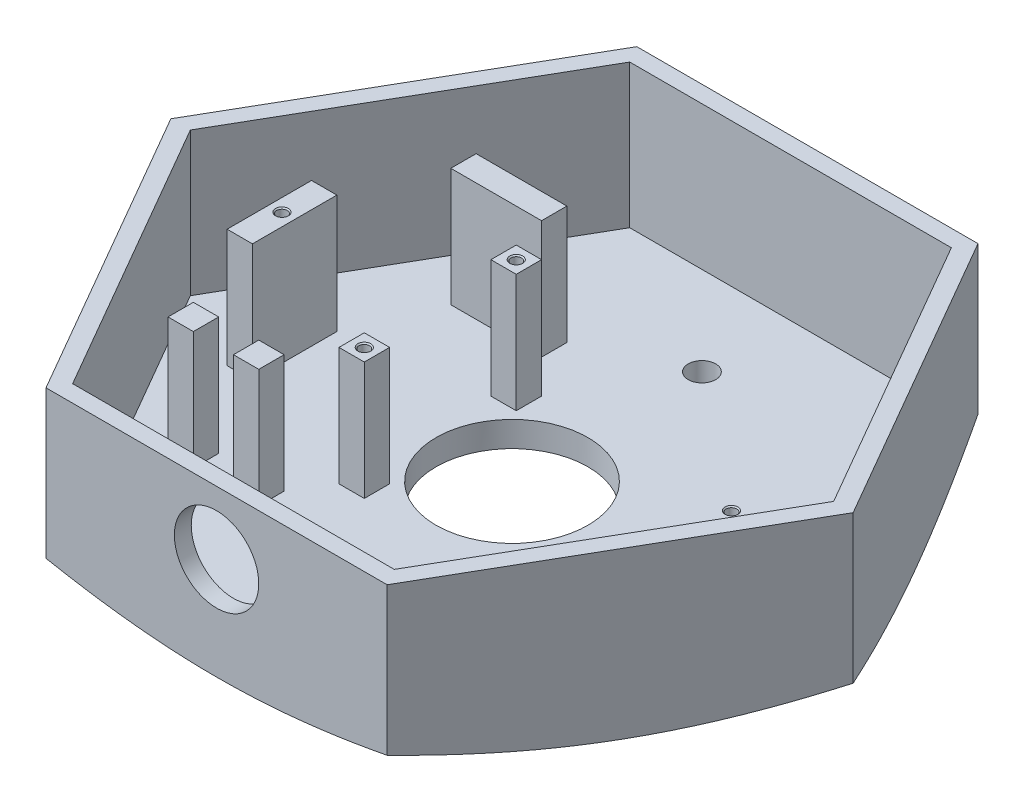
from build123d import *

# Parameters (mm, degrees)
BOSS_EXTRUDE1_DEPTH         = 41
CUT_EXTRUDE1_DEPTH          = 34
SKETCH4_R                   = 52.5
CUT_EXTRUDE2_DEPTH          = 1
SKETCH5_W                   = 21.5
SKETCH5_H                   = 6
SKETCH5_W_2                 = 6
SKETCH5_H_2                 = 20
BOSS_EXTRUDE2_DEPTH         = 28
SKETCH6_R                   = 18
CUT_EXTRUDE3_DEPTH          = 28
SKETCH7_R                   = 3.25
CUT_EXTRUDE4_DEPTH          = 28
M3_TAPPED_HOLE1_D           = 2.5
M3_TAPPED_HOLE1_CSINK_D     = 3.05
M3_TAPPED_HOLE1_CSINK_ANGLE = 90
M3_TAPPED_HOLE2_D           = 2.5
M3_TAPPED_HOLE2_DEPTH       = 8
M3_TAPPED_HOLE2_CSINK_D     = 3.05
M3_TAPPED_HOLE2_CSINK_ANGLE = 90
M3_TAPPED_HOLE2_TIP         = 0.751075774
SKETCH8_R                   = 10
CUT_EXTRUDE5_DEPTH          = 28


with BuildPart() as part:
    # Sketch1 → Boss-Extrude1 (new body)
    with BuildSketch(Plane(origin=(0, 0, 0), x_dir=(1, 0, 0), z_dir=(0, 1, 0))):
        Polygon((-40.414518843, 70), (-80.829037687, 0), (-40.414518843, -70), (40.414518843, -70), (80.829037687, 0), (40.414518843, 70), align=None)
    extrude(amount=BOSS_EXTRUDE1_DEPTH)

    # Sketch2 → Cut-Extrude1 (cut)
    with BuildSketch(Plane(origin=(0, 41, 0), x_dir=(1, 0, 0), z_dir=(0, 1, 0))):
        Polygon((38.105117767, -66), (76.210235533, 0), (38.105117767, 66), (-38.105117767, 66), (-76.210235533, 0), (-38.105117767, -66), align=None)
    extrude(amount=-CUT_EXTRUDE1_DEPTH, mode=Mode.SUBTRACT)

    # Sketch3 → Cut-Revolve1 (revolve, cut)
    with BuildSketch(Plane.XY, mode=Mode.PRIVATE) as cut_revolve1_sk:
        Polygon((-80.829037687, 6), (-65.198503298, 0), (-80.829037687, 0), align=None)
    revolve(cut_revolve1_sk.sketch.rotate(Axis((0, 62.900603769, 0), (0, -1, 0)), 270), axis=Axis((0, 62.900603769, 0), (0, -1, 0)), mode=Mode.SUBTRACT)

    # Sketch4 → Cut-Extrude2 (cut)
    with BuildSketch(Plane.XZ):
        with Locations(Location((0, 0, 0), (0, 0, 270))):
            Circle(SKETCH4_R)
    extrude(amount=-CUT_EXTRUDE2_DEPTH, mode=Mode.SUBTRACT)

    # Sketch5 → Boss-Extrude2 (add)
    with BuildSketch(Plane(origin=(0, 7, 0), x_dir=(1, 0, 0), z_dir=(0, 1, 0))):
        with Locations((-32.75, 32)):
            Rectangle(SKETCH5_W, SKETCH5_H)
        with Locations((-54.5, 0)):
            Rectangle(SKETCH5_W_2, SKETCH5_H_2)
        with Locations((-43.5, -32)):
            Rectangle(SKETCH5_W_2, SKETCH5_H)
        with Locations((-28, -32)):
            Rectangle(SKETCH5_W_2, SKETCH5_H)
        with Locations((-17, 18)):
            Rectangle(SKETCH5_W_2, SKETCH5_H)
        with Locations((-17, -18)):
            Rectangle(SKETCH5_W_2, SKETCH5_H)
    extrude(amount=BOSS_EXTRUDE2_DEPTH)

    # Sketch6 → Cut-Extrude3 (cut)
    with BuildSketch(Plane(origin=(0, 7, 0), x_dir=(1, 0, 0), z_dir=(0, 1, 0))):
        with Locations(Location((0, 0, 0), (0, 0, 270))):
            Circle(SKETCH6_R)
    extrude(amount=-CUT_EXTRUDE3_DEPTH, mode=Mode.SUBTRACT)

    # Sketch7 → Cut-Extrude4 (cut)
    with BuildSketch(Plane(origin=(0, 7, 0), x_dir=(1, 0, 0), z_dir=(0, 1, 0))):
        with Locations(Location((0, 45, 0), (0, 0, 270))):
            Circle(SKETCH7_R)
        with Locations(Location((0, -45, 0), (0, 0, 90))):
            Circle(SKETCH7_R)
    extrude(amount=-CUT_EXTRUDE4_DEPTH, mode=Mode.SUBTRACT)

    # M3 Tapped Hole1 (through all)
    with Locations(Plane(origin=(0, 7, 0), x_dir=(1, 0, 0), z_dir=(0, 1, 0))):
        with Locations((32, 20), (32, -20)):
            CounterSinkHole(M3_TAPPED_HOLE1_D / 2, M3_TAPPED_HOLE1_CSINK_D / 2, counter_sink_angle=M3_TAPPED_HOLE1_CSINK_ANGLE)

    # M3 Tapped Hole2
    with Locations(Plane(origin=(0, 35, 0), x_dir=(1, 0, 0), z_dir=(0, 1, 0))):
        with Locations((-54.5, 0), (-17, 18), (-17, -18)):
            CounterSinkHole(M3_TAPPED_HOLE2_D / 2, M3_TAPPED_HOLE2_CSINK_D / 2, depth=M3_TAPPED_HOLE2_DEPTH, counter_sink_angle=M3_TAPPED_HOLE2_CSINK_ANGLE)
            with Locations((0, 0, -(M3_TAPPED_HOLE2_DEPTH + M3_TAPPED_HOLE2_TIP / 2))):  # 118° drill point
                Cone(0, M3_TAPPED_HOLE2_D / 2, M3_TAPPED_HOLE2_TIP, mode=Mode.SUBTRACT)

    # Sketch8 → Cut-Extrude5 (cut)
    with BuildSketch(Plane(origin=(0, 0, 66), x_dir=(-1, 0, 0), z_dir=(0, 0, -1))):
        with Locations((0, 26)):
            Circle(SKETCH8_R)
    extrude(amount=-CUT_EXTRUDE5_DEPTH, mode=Mode.SUBTRACT)


solid = part.part
